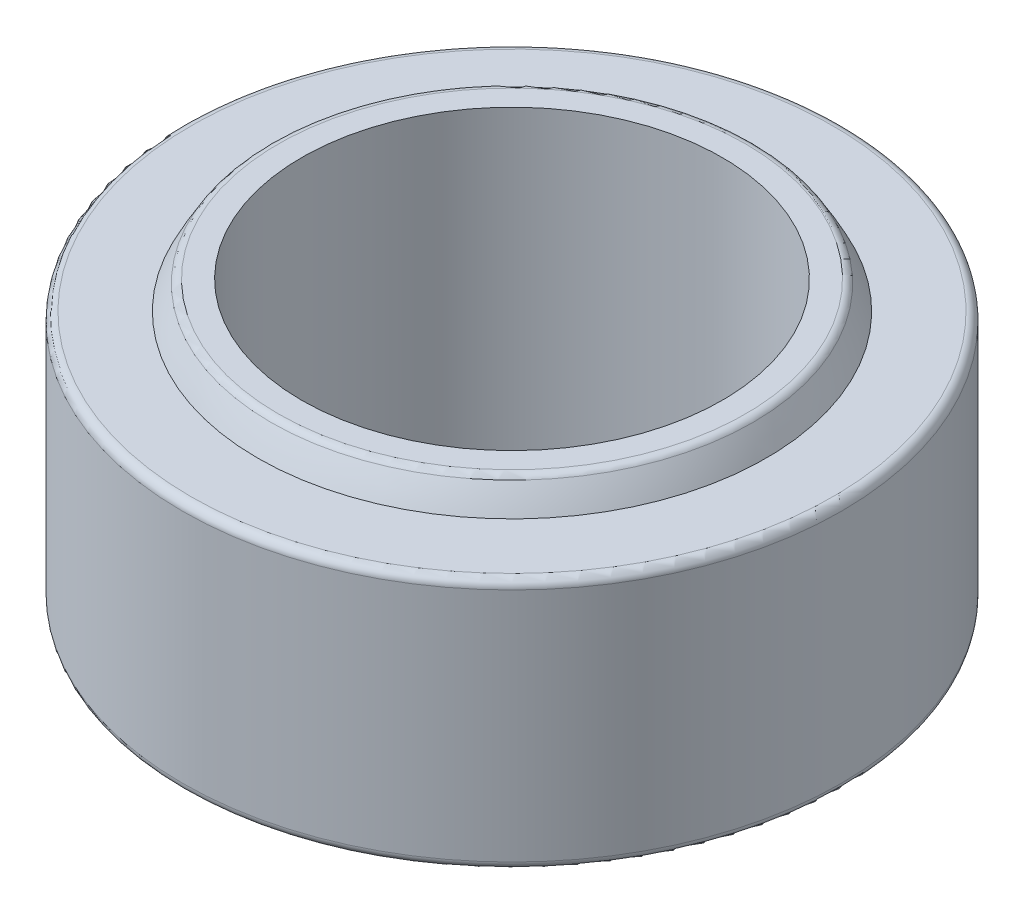
SolidWorks part; units mm, degrees
ref_plane "前视基准面" through (0, 0, 0) normal (0, 0, 1) x (1, 0, 0)
ref_plane "上视基准面" through (0, 0, 0) normal (0, 1, 0) x (1, 0, 0)
ref_plane "右视基准面" through (0, 0, 0) normal (1, 0, 0) x (0, 0, -1)
sketch "草图1" plane through (0, 0, 0) normal (1, 0, 0) x (0, 0, -1)
  line L0 (-23.5, 0) -> (23.5, 0) construction
  line L1 (0, 11) -> (0, -11) construction
  line L2 (-23.5, -8.4) -> (-23.5, 8.4)
  line L3 (-22.9, 9) -> (-18.1384, 9)
  line L4 (-22.9, -9) -> (-18.1384, -9)
  line L5 (22.9, -9) -> (18.1384, -9)
  line L6 (23.5, -8.4) -> (23.5, 8.4)
  line L7 (22.9, 9) -> (18.1384, 9)
  line L8 (-16.6704, 11) -> (16.6704, 11)
  line L9 (-16.6704, -11) -> (16.6704, -11)
  line L10 (-15, 11) -> (-15, -11)
  line L15 (-2.1165, 20.1375) -> (0, 0)
  line L16 (2.1165, 20.1375) -> (0, 0)
  line L18 (-2.1165, 20.1375) -> (2.1165, 20.1375) construction
  arc A0 (-17.1794, 10.7176) -> (-17.1794, -10.7176) centre (0, 0) ccw
  arc A1 (17.1794, -10.7176) -> (17.1794, 10.7176) centre (0, 0) ccw
  arc A2 (-16.6704, -11) -> (-17.1794, -10.7176) centre (-16.6704, -10.4) cw
  arc A3 (2.1165, 20.1375) -> (-2.1165, 20.1375) centre (0, 0) ccw
  circle A4 centre (0, 0) radius 20.2485 construction
  arc A5 (16.6704, -11) -> (17.1794, -10.7176) centre (16.6704, -10.4) ccw
  arc A6 (16.6704, 11) -> (17.1794, 10.7176) centre (16.6704, 10.4) cw
  arc A7 (-16.6704, 11) -> (-17.1794, 10.7176) centre (-16.6704, 10.4) ccw
  arc A8 (22.9, -9) -> (23.5, -8.4) centre (22.9, -8.4) ccw
  arc A9 (23.5, 8.4) -> (22.9, 9) centre (22.9, 8.4) ccw
  arc A10 (-22.9, -9) -> (-23.5, -8.4) centre (-22.9, -8.4) cw
  arc A11 (-23.5, 8.4) -> (-22.9, 9) centre (-22.9, 8.4) cw
  point P23 (-17, -11)
  point P26 (17, -11)
  point P34 (17, 11)
  point P37 (-17, 11)
  point P40 (23.5, -9)
  point P43 (23.5, 9)
  point P46 (-23.5, -9)
  point P49 (-23.5, 9)
  dimension "r1" = 0.6
  dimension "r2" = 0.6
  dimension "C" = 18
  dimension "D" = 47
  dimension "B" = 22
  dimension "(d1)" = 34
  dimension "(d)" = 30
  dimension "a" = 6
sketch "草图2" plane through (0, 0, 0) normal (1, 0, 0) x (0, 0, -1)
  line L2 (-22.9, -9) -> (-18.1384, -9) construction
  line L3 (-22.9, 9) -> (-18.1384, 9)
  line L4 (-23.5, -8.4) -> (-23.5, 8.4) construction
  line L5 (-22.9, -9) -> (-18.1384, -9)
  line L6 (-23.5, -8.4) -> (-23.5, 8.4)
  arc A0 (-17.1794, 10.7176) -> (-17.1794, -10.7176) centre (0, 0) ccw construction
  arc A1 (-18.1384, 9) -> (-18.1384, -9) centre (0, 0) ccw
  arc A2 (-22.9, 9) -> (-23.5, 8.4) centre (-22.9, 8.4) ccw construction
  arc A3 (-23.5, -8.4) -> (-22.9, -9) centre (-22.9, -8.4) ccw construction
  arc A4 (-22.9, 9) -> (-23.5, 8.4) centre (-22.9, 8.4) ccw
  arc A5 (-23.5, -8.4) -> (-22.9, -9) centre (-22.9, -8.4) ccw
revolve "旋转1" add sketch "草图2" angle 360 about L1
sketch "草图3" plane through (0, 0, 0) normal (1, 0, 0) x (0, 0, -1)
  line L0 (-16.6704, 11) -> (16.6704, 11) construction
  line L1 (-15, 11) -> (-15, -11) construction
  line L2 (-16.6704, -11) -> (16.6704, -11) construction
  line L3 (-16.6704, 11) -> (-15, 11)
  line L4 (-15, 11) -> (-15, -11)
  line L5 (-16.6704, -11) -> (-15, -11)
  arc A0 (-16.6704, 11) -> (-17.1794, 10.7176) centre (-16.6704, 10.4) ccw construction
  arc A1 (-17.1794, 10.7176) -> (-17.1794, -10.7176) centre (0, 0) ccw construction
  arc A2 (-17.1794, -10.7176) -> (-16.6704, -11) centre (-16.6704, -10.4) ccw construction
  arc A3 (-16.6704, 11) -> (-17.1794, 10.7176) centre (-16.6704, 10.4) ccw
  arc A4 (-17.1794, 10.7176) -> (-17.1794, -10.7176) centre (0, 0) ccw
  arc A5 (-17.1794, -10.7176) -> (-16.6704, -11) centre (-16.6704, -10.4) ccw
revolve "旋转2" add sketch "草图3" angle 360 about L1
